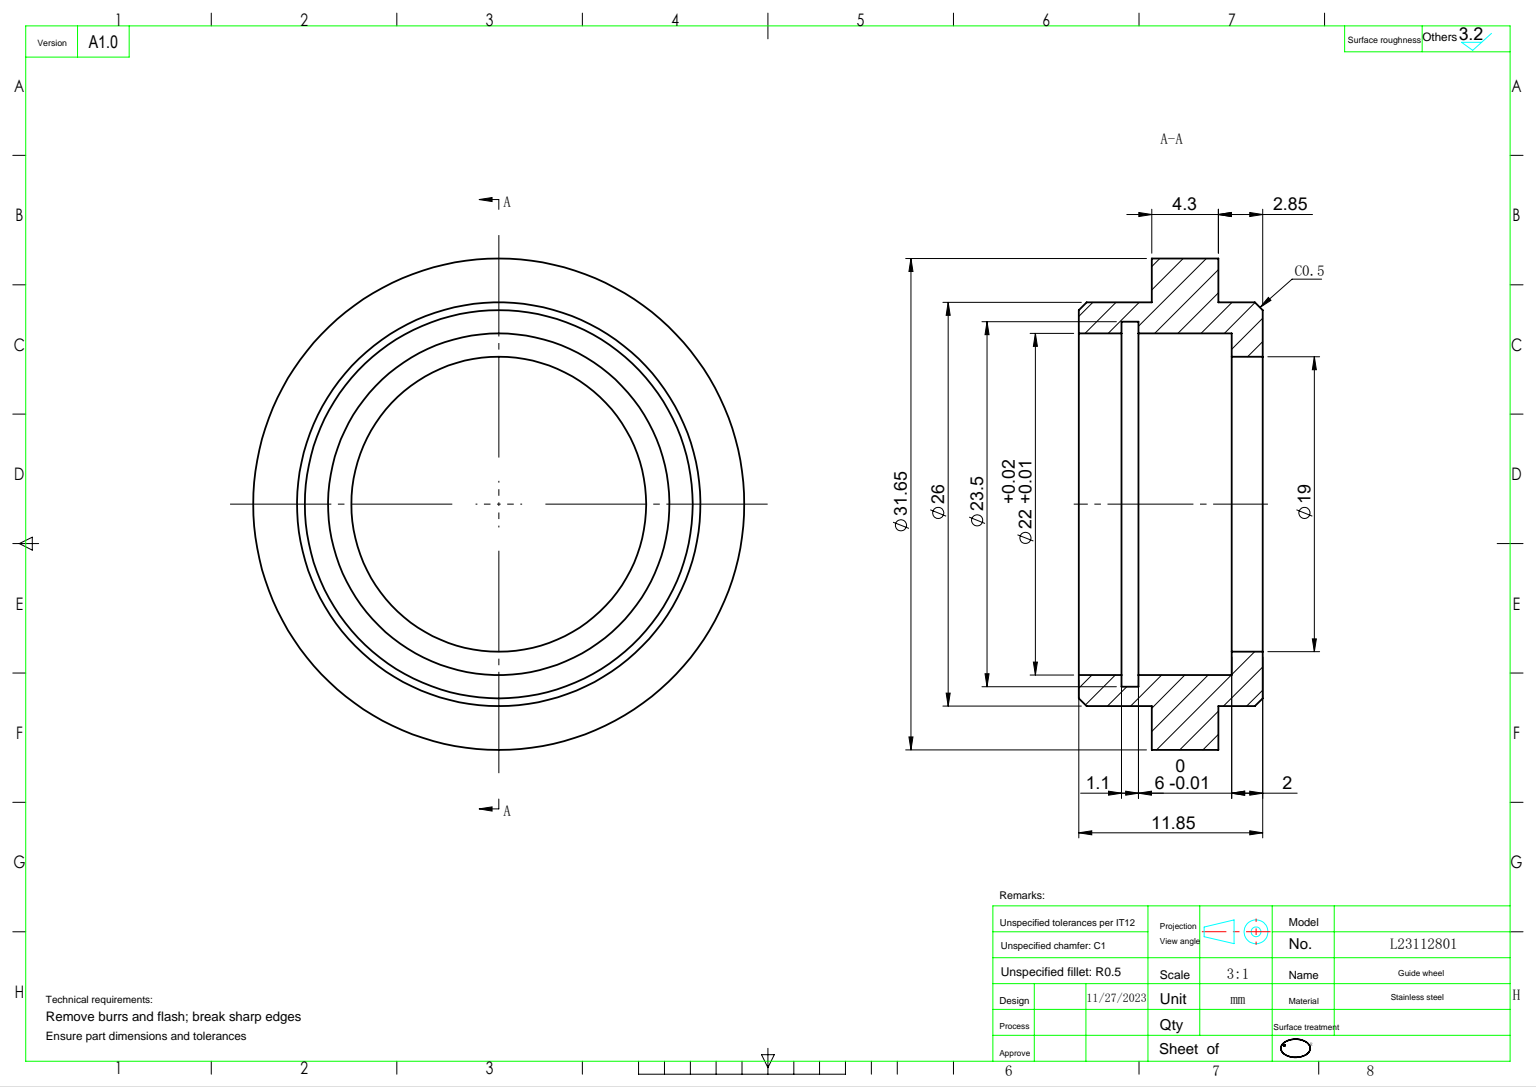
from build123d import *

# Parameters (mm, degrees)
CUT_EXTRUDE_START   = 2
SKETCH_2_R          = 11
CUT_EXTRUDE_1_DEPTH = 24.323580908
CUT_EXTRUDE_START_2 = 6
SKETCH_3_R          = 11.75
CUT_EXTRUDE_2_DEPTH = 1.1
CHAMFER_1_SIZE      = 0.5


with BuildPart() as part:
    # 草图1 → 旋转1 (revolve)
    with BuildSketch(Plane.XY, mode=Mode.PRIVATE) as revolve_1_sk:
        Polygon((0, 9.5), (0, 13), (2.85, 13), (2.85, 15.825), (7.15, 15.825), (7.15, 13), (11.85, 13), (11.85, 9.5), align=None)
    revolve(revolve_1_sk.sketch.rotate(Axis((0, 0, 0), (1, 0, 0)), 90), axis=Axis((0, 0, 0), (1, 0, 0)))

    # 草图2 → 切除-拉伸1 (cut, through all)
    with BuildSketch(Plane(origin=(0, 0, 0), x_dir=(0, 0, -1), z_dir=(1, 0, 0)).offset(CUT_EXTRUDE_START)):
        Circle(SKETCH_2_R)
    extrude(amount=CUT_EXTRUDE_1_DEPTH, mode=Mode.SUBTRACT)

    # 草图3 → 切除-拉伸2 (cut)
    with BuildSketch(Plane(origin=(2, 0, 0), x_dir=(0, 0, -1), z_dir=(1, 0, 0)).offset(CUT_EXTRUDE_START_2)):
        Circle(SKETCH_3_R)
    extrude(amount=CUT_EXTRUDE_2_DEPTH, mode=Mode.SUBTRACT)

    # 倒角1
    chamfer_1_edges = [part.edges().sort_by_distance(p)[0] for p in [
        (11.85, 0, -13),
        (0, 0, -13),
    ]]
    chamfer(chamfer_1_edges, length=CHAMFER_1_SIZE)


solid = part.part
